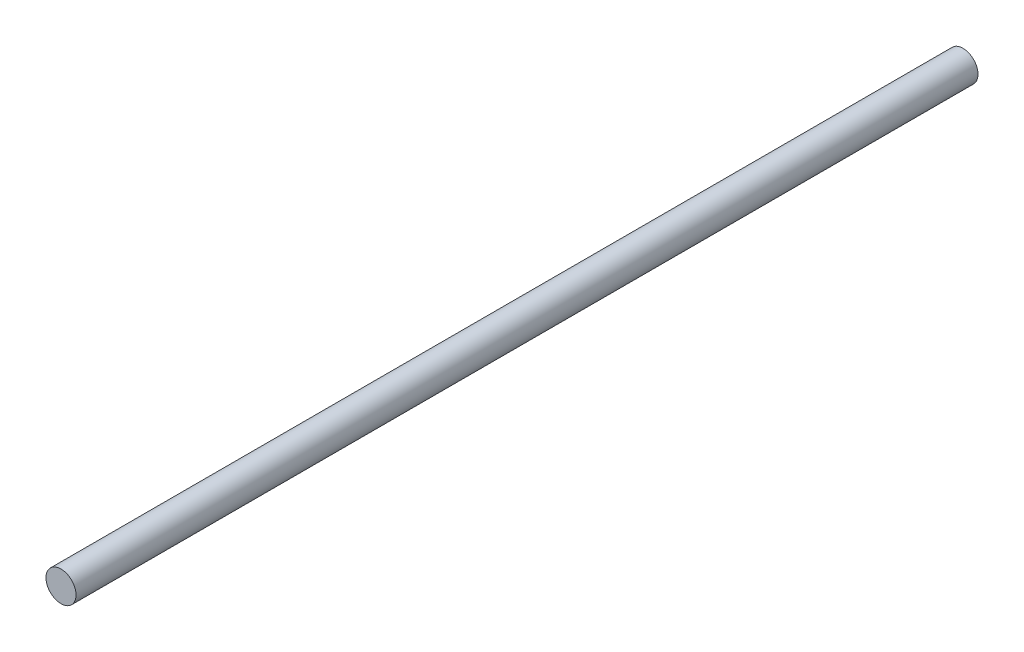
SolidWorks part; units mm, degrees
ref_plane "Front Plane" through (0, 0, 0) normal (0, 0, 1) x (1, 0, 0)
ref_plane "Top Plane" through (0, 0, 0) normal (0, 1, 0) x (1, 0, 0)
ref_plane "Right Plane" through (0, 0, 0) normal (1, 0, 0) x (0, 0, -1)
sketch "Sketch1" plane through (0, 0, 0) normal (0, 0, 1) x (1, 0, 0)
  circle A0 centre (0, 0) radius 1
  dimension "D1" = 2
extrude "Boss-Extrude1" add sketch "Sketch1" along normal blind 60
